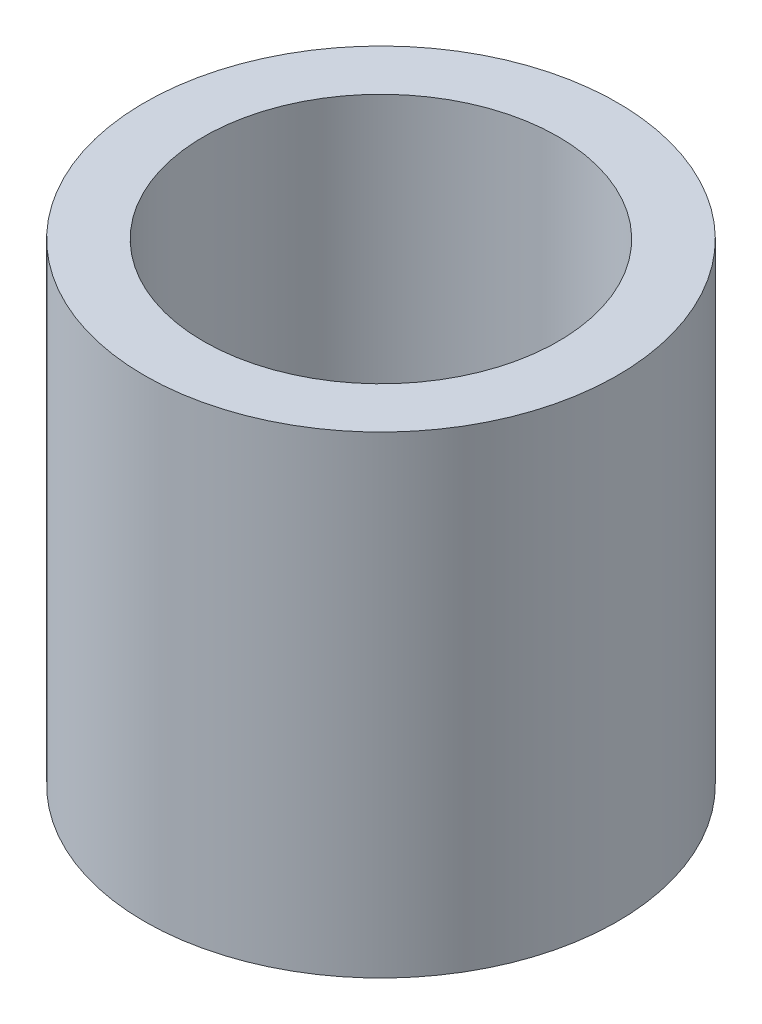
from build123d import *

# Parameters (mm, degrees)
SKETCH_1_R      = 4
SKETCH_1_R_2    = 3
EXTRUDE_1_DEPTH = 8


with BuildPart() as part:
    # 草图1 → 凸台-拉伸1 (new body)
    with BuildSketch(Plane(origin=(0, 0, 0), x_dir=(1, 0, 0), z_dir=(0, 1, 0))):
        with Locations(Location((0, 0, 0), (0, 0, 270))):
            Circle(SKETCH_1_R)
        with Locations(Location((0, 0, 0), (0, 0, 270))):
            Circle(SKETCH_1_R_2, mode=Mode.SUBTRACT)
    extrude(amount=EXTRUDE_1_DEPTH)


solid = part.part
